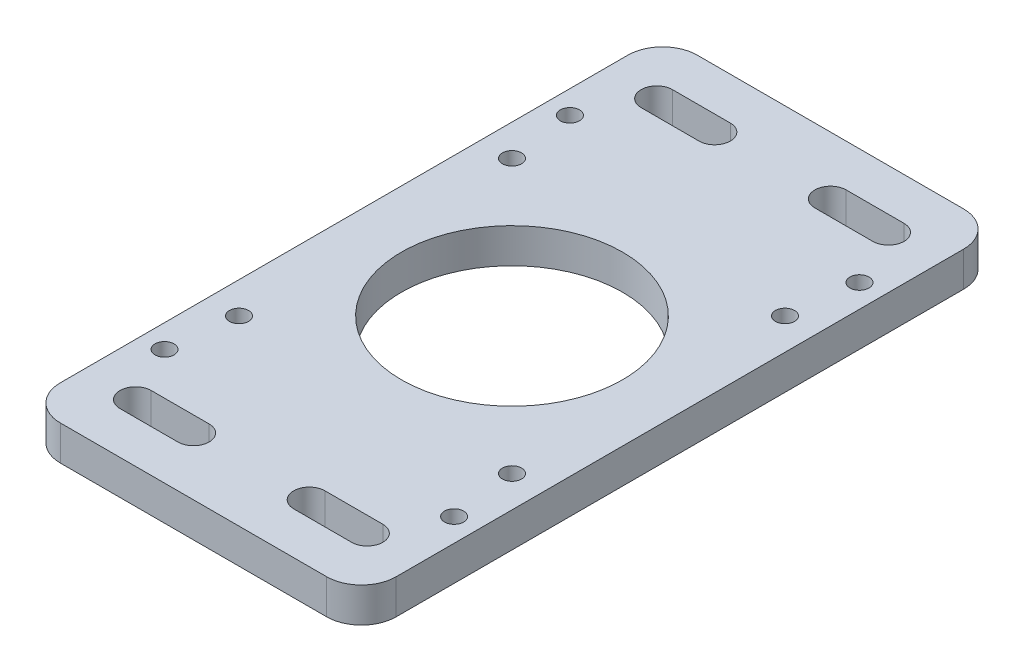
SolidWorks part; units mm, degrees
material "Q235"
ref_plane "Front Plane" through (0, 0, 0) normal (0, 0, 1) x (1, 0, 0)
ref_plane "Top Plane" through (0, 0, 0) normal (0, 1, 0) x (1, 0, 0)
ref_plane "Right Plane" through (0, 0, 0) normal (1, 0, 0) x (0, 0, -1)
sketch "Sketch1" plane through (0, 0, 0) normal (0, 1, 0) x (1, 0, 0)
  line L1 (-23, 55) -> (23, 55)
  line L2 (-29, 49) -> (-29, -49)
  line L3 (-23, -55) -> (23, -55)
  line L4 (29, 49) -> (29, -49)
  line L5 (-29, 55) -> (29, -55) construction
  line L6 (-29, -55) -> (29, 55) construction
  circle A0 centre (0, 0) radius 19.1
  arc A1 (23, 55) -> (29, 49) centre (23, 49) cw
  arc A2 (-23, 55) -> (-29, 49) centre (-23, 49) ccw
  arc A3 (-29, -49) -> (-23, -55) centre (-23, -49) ccw
  arc A4 (23, -55) -> (29, -49) centre (23, -49) ccw
  point P0 (0, 0)
  dimension "D3" = 38.2
  dimension "D4" = 6
  dimension "D1" = 58
  dimension "D2" = 110
extrude "Boss-Extrude1" add sketch "Sketch1" along normal blind 6
hole_wizard "M4 Tapped Hole1" positions "Sketch2" profile "Sketch3" tap size "M4" standard "GB"
sketch "Sketch2" plane through (0, 6, 0) normal (0, 1, 0) x (1, 0, 0)
  line L0 (-23.57, 23.57) -> (-23.57, -23.57)
  line L1 (-23.57, -23.57) -> (23.57, -23.57)
  line L2 (23.57, -23.57) -> (23.57, 23.57)
  line L3 (23.57, 23.57) -> (-23.57, 23.57)
  line L5 (0, 23.57) -> (0, 0)
  line L6 (0, 0) -> (23.57, 0)
  point P0 (-23.57, 23.57)
  point P2 (23.57, 23.57)
  point P4 (23.57, -23.57)
  point P6 (-23.57, -23.57)
  dimension "D1" = 47.14
sketch "Sketch3" plane through (-23.57, 6, -23.57) normal (1, 0, 0) x (0, 0, 1)
  line L0 (0, 0) -> (0, 11.0914)
  line L1 (0, 11.0914) -> (1.65, 10.1)
  line L2 (1.65, 10.1) -> (1.65, 0)
  line L5 (1.65, 0) -> (0, 0)
  line L10 (0, 11.0914) -> (-1.65, 10.1) construction
  line L11 (0, -6.35) -> (0, 107.95) construction
  dimension "螺纹孔钻头直径" = 3.3
  dimension "螺纹孔钻头深度" = 10.1
  dimension "导头角度" = 118
cosmetic thread "Hole Thread1" parameters "D1"=8, "D2"=4
cosmetic thread "Hole Thread2" parameters "D1"=8, "D2"=4
cosmetic thread "Hole Thread3" parameters "D1"=8, "D2"=4
cosmetic thread "Hole Thread4" parameters "D1"=8, "D2"=4
sketch "Sketch4" plane through (0, 0, 0) normal (0, -1, 0) x (1, 0, 0)
  line L0 (-20, 45) -> (-10, 45) construction
  line L1 (-20, 47.7) -> (-10, 47.7)
  line L2 (-20, 42.3) -> (-10, 42.3)
  line L3 (20, 45) -> (10, 45) construction
  line L6 (0, 15.975) -> (0, 0) construction
  line L7 (0, 0) -> (35.6111, 0) construction
  line L8 (20, 47.7) -> (10, 47.7)
  line L9 (20, 42.3) -> (10, 42.3)
  line L10 (-20, -45) -> (-10, -45) construction
  line L11 (-20, -47.7) -> (-10, -47.7)
  line L12 (-20, -42.3) -> (-10, -42.3)
  line L13 (20, -45) -> (10, -45) construction
  line L14 (20, -47.7) -> (10, -47.7)
  line L15 (20, -42.3) -> (10, -42.3)
  arc A0 (-20, 47.7) -> (-20, 42.3) centre (-20, 45) ccw
  arc A1 (-10, 42.3) -> (-10, 47.7) centre (-10, 45) ccw
  arc A4 (20, 47.7) -> (20, 42.3) centre (20, 45) cw
  arc A5 (10, 42.3) -> (10, 47.7) centre (10, 45) cw
  arc A6 (-20, -47.7) -> (-20, -42.3) centre (-20, -45) cw
  arc A7 (-10, -42.3) -> (-10, -47.7) centre (-10, -45) cw
  arc A8 (20, -47.7) -> (20, -42.3) centre (20, -45) ccw
  arc A9 (10, -42.3) -> (10, -47.7) centre (10, -45) ccw
  point P2 (-15, 45)
  point P9 (15, 45)
  point P21 (-15, -45)
  point P28 (15, -45)
  dimension "D3" = 2.7
  dimension "D1" = 30
  dimension "D2" = 45
  dimension "D4" = 10
extrude "Cut-Extrude1" cut sketch "Sketch4" against normal through all
hole_wizard "M4 Tapped Hole2" positions "Sketch5" profile "Sketch6" tap size "M4" standard "GB"
sketch "Sketch5" plane through (0, 0, 0) normal (0, -1, 0) x (-1, 0, 0)
  line L0 (-25, -35) -> (25, -35)
  line L1 (25, -35) -> (25, 35)
  line L2 (25, 35) -> (-25, 35)
  line L3 (-25, 35) -> (-25, -35)
  line L5 (0, -35) -> (0, 0)
  line L6 (0, 0) -> (25, 0)
  point P0 (25, -35)
  point P2 (25, 35)
  point P4 (-25, 35)
  point P6 (-25, -35)
  dimension "D1" = 70
  dimension "D2" = 50
sketch "Sketch6" plane through (-25, 0, 35) normal (1, 0, 0) x (0, 0, -1)
  line L0 (0, 0) -> (0, 11.0914)
  line L1 (0, 11.0914) -> (1.65, 10.1)
  line L2 (1.65, 10.1) -> (1.65, 0)
  line L5 (1.65, 0) -> (0, 0)
  line L10 (0, 11.0914) -> (-1.65, 10.1) construction
  line L11 (0, -6.35) -> (0, 107.95) construction
  dimension "螺纹孔钻头直径" = 3.3
  dimension "螺纹孔钻头深度" = 10.1
  dimension "导头角度" = 118
cosmetic thread "Hole Thread5" parameters "D1"=8, "D2"=4
cosmetic thread "Hole Thread6" parameters "D1"=8, "D2"=4
cosmetic thread "Hole Thread7" parameters "D1"=8, "D2"=4
cosmetic thread "Hole Thread8" parameters "D1"=8, "D2"=4
